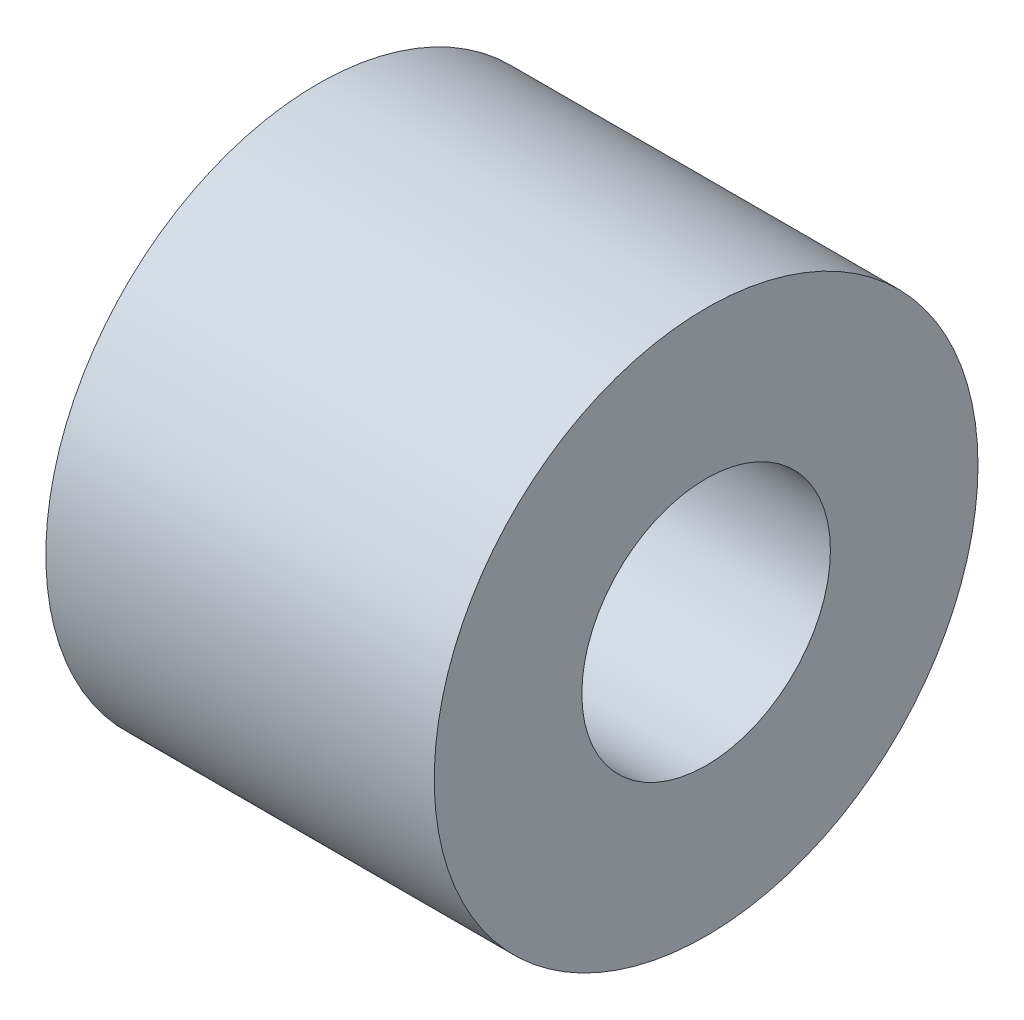
SolidWorks part; units mm, degrees
material "ABS"
ref_plane "前视基准面" through (0, 0, 0) normal (0, 0, 1) x (1, 0, 0)
ref_plane "上视基准面" through (0, 0, 0) normal (0, 1, 0) x (1, 0, 0)
ref_plane "右视基准面" through (0, 0, 0) normal (1, 0, 0) x (0, 0, -1)
other "Configuration Table"
sketch "草图1" plane through (0, 0, 0) normal (1, 0, 0) x (0, 0, -1)
  circle A0 centre (0, 0) radius 1.6
  circle A1 centre (0, 0) radius 3.5
  dimension "D1" = 3.2
  dimension "D2" = 7
extrude "凸台-拉伸1" add sketch "草图1" along normal blind 5
